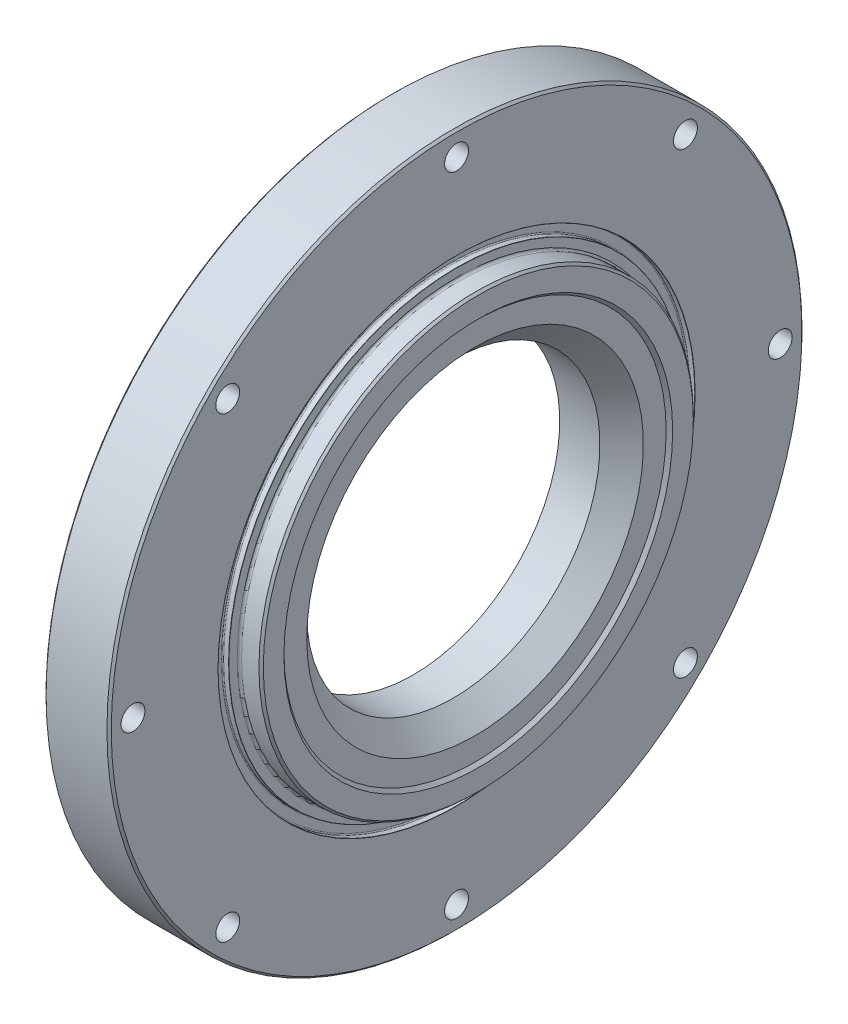
SolidWorks part; units mm, degrees
material "1.6571 (20NiCrMoS6-4)"
ref_plane "Front Plane" through (0, 0, 0) normal (0, 0, 1) x (1, 0, 0)
ref_plane "Top Plane" through (0, 0, 0) normal (0, 1, 0) x (1, 0, 0)
ref_plane "Right Plane" through (0, 0, 0) normal (1, 0, 0) x (0, 0, -1)
sketch "Sketch1" plane through (0, 0, 0) normal (0, 0, 1) x (1, 0, 0)
  line L0 (0, 0) -> (287.7519, 0) construction
  line L1 (0, 273.05) -> (0, 320)
  line L2 (0, 320) -> (60, 320)
  line L3 (60, 320) -> (60, 219.7)
  line L4 (60, 200) -> (80, 200)
  line L5 (80, 200) -> (80, 179)
  line L6 (80, 179) -> (77, 176)
  line L7 (57, 135) -> (20, 135)
  line L8 (20, 135) -> (20, 234.6)
  line L9 (20, 273.05) -> (0, 273.05)
  line L10 (77, 176) -> (77, 155)
  line L11 (77, 155) -> (57, 135)
  line L12 (20.2, 244.5) -> (24.72, 244.5)
  line L13 (25.72, 243.5) -> (25.72, 235.8)
  line L14 (24.72, 234.8) -> (20.2, 234.8)
  line L15 (20, 244.7) -> (20, 273.05)
  line L16 (59.8, 219.5) -> (55.28, 219.5)
  line L17 (54.28, 218.5) -> (54.28, 210.8)
  line L18 (55.28, 209.8) -> (59.8, 209.8)
  line L19 (60, 209.6) -> (60, 200)
  arc A0 (25.72, 235.8) -> (24.72, 234.8) centre (24.72, 235.8) cw
  arc A1 (24.72, 244.5) -> (25.72, 243.5) centre (24.72, 243.5) cw
  arc A2 (20.2, 234.8) -> (20, 234.6) centre (20.2, 234.6) ccw
  arc A3 (20.2, 244.5) -> (20, 244.7) centre (20.2, 244.7) cw
  arc A4 (59.8, 209.8) -> (60, 209.6) centre (59.8, 209.6) cw
  arc A5 (59.8, 219.5) -> (60, 219.7) centre (59.8, 219.7) ccw
  arc A6 (54.28, 210.8) -> (55.28, 209.8) centre (55.28, 210.8) ccw
  arc A7 (55.28, 219.5) -> (54.28, 218.5) centre (55.28, 218.5) ccw
  point P26 (20, 244.5)
  point P33 (60, 209.8)
  dimension "D16" = 1
  dimension "D17" = 0.2
  dimension "D21" = 0.2
  dimension "D22" = 1
  dimension "D1" = 320
  dimension "D2" = 273.05
  dimension "D3" = 20
  dimension "D4" = 40
  dimension "D5" = 20
  dimension "D6" = 3
  dimension "D7" = 200
  dimension "D8" = 135
  dimension "D9" = 21
  dimension "D10" = 20
  dimension "D11" = 45
  dimension "D12" = 45
  dimension "D13" = 5.72
  dimension "D14" = 9.7
  dimension "D15" = 244.5
  dimension "D18" = 5.72
  dimension "D19" = 9.7
  dimension "D20" = 219.5
revolve "Revolve1" add sketch "Sketch1" angle 360 about L0
fillet "Fillet1" radius 2 1 edges at (20, 0, 273.05)
chamfer "Chamfer1" distance 2 angle 45 3 edges at (60, 0, 320) (0, 0, 273.05) (0, 0, 320)
fillet "Fillet2" radius 2 1 edges at (60, 0, 200)
chamfer "Chamfer2" distance 2 angle 45 1 edges at (80, 0, 200)
sketch "Sketch2" plane through (0, 0, 0) normal (-1, 0, 0) x (0, 0, 1)
  line L0 (0, 0) -> (0, 298) construction
  circle A0 centre (0, 0) radius 298 construction
  circle A1 centre (0, 298) radius 11
  circle A2 centre (210.7178, 210.7178) radius 11
  circle A3 centre (298, 0) radius 11
  circle A4 centre (210.7178, -210.7178) radius 11
  circle A5 centre (0, -298) radius 11
  circle A6 centre (-210.7178, -210.7178) radius 11
  circle A7 centre (-298, 0) radius 11
  circle A8 centre (-210.7178, 210.7178) radius 11
  point P22 (0, 0)
  dimension "D1" = 596
  dimension "D2" = 22
  dimension "D3" = 8
extrude "Cut-Extrude1" cut sketch "Sketch2" against normal through all
sketch "Sketch3" plane through (0, 0, 0) normal (-1, 0, 0) x (0, 0, 1)
  circle A0 centre (0, 0) radius 298 construction
  circle A1 centre (0, 298) radius 16.5
  circle A2 centre (210.7178, 210.7178) radius 16.5
  circle A3 centre (298, 0) radius 16.5
  circle A4 centre (210.7178, -210.7178) radius 16.5
  circle A5 centre (0, -298) radius 16.5
  circle A6 centre (-210.7178, -210.7178) radius 16.5
  circle A7 centre (-298, 0) radius 16.5
  circle A8 centre (-210.7178, 210.7178) radius 16.5
  point P23 (0, 0)
  dimension "D1" = 33
  dimension "D2" = 8
extrude "Cut-Extrude2" cut sketch "Sketch3" against normal blind 35
